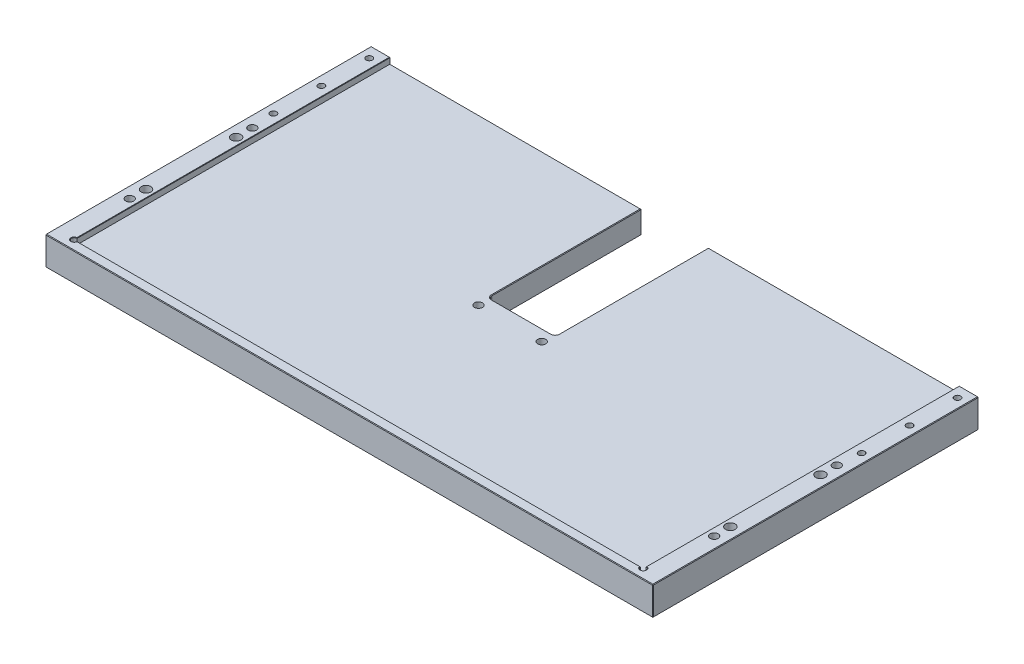
from build123d import *

# Parameters (mm, degrees)
SKETCH_1_W             = 317
SKETCH_1_H             = 170
EXTRUDE_1_DEPTH        = 15
SKETCH_2_W             = 297
SKETCH_2_H             = 330
CUT_EXTRUDE_1_DEPTH    = 3.1
SKETCH_3_W             = 35
SKETCH_3_H             = 103.554222687
CUT_EXTRUDE_2_DEPTH    = 181.477837975
HOLE_WIZARD_M5_1_D     = 4.2
HOLE_WIZARD_M5_1_DEPTH = 16
HOLE_WIZARD_M5_1_TIP   = 1.2618073
FILLET_1_R             = 2
SKETCH_6_R             = 1.5
CUT_EXTRUDE_3_DEPTH    = 5
CHAMFER_1_SIZE         = 0.3
HOLE_WIZARD_M5_2_D     = 4.2
HOLE_WIZARD_M4_1_D     = 3.3
HOLE_WIZARD_M4_1_DEPTH = 13.5
HOLE_WIZARD_M4_1_TIP   = 0.991420021
SKETCH_11_R            = 2.5
CUT_EXTRUDE_4_DEPTH    = 10
SKETCH_12_R            = 1.5
CUT_EXTRUDE_5_DEPTH    = 181.477837975
HOLE_WIZARD_M4_2_D     = 3.3
HOLE_WIZARD_M4_2_DEPTH = 9
HOLE_WIZARD_M4_2_TIP   = 0.991420021
CHAMFER_3_SIZE         = 0.2


with BuildPart() as part:
    # 草图1 → 凸台-拉伸1 (new body)
    with BuildSketch(Plane(origin=(0, 0, 0), x_dir=(1, 0, 0), z_dir=(0, 1, 0))):
        Rectangle(SKETCH_1_W, SKETCH_1_H)
    extrude(amount=EXTRUDE_1_DEPTH)

    # 草图2 → 切除-拉伸1 (cut)
    with BuildSketch(Plane(origin=(0, 15, 0), x_dir=(1, 0, 0), z_dir=(0, 1, 0))):
        with Locations((0, 85)):
            Rectangle(SKETCH_2_W, SKETCH_2_H)
    extrude(amount=-CUT_EXTRUDE_1_DEPTH, mode=Mode.SUBTRACT)

    # 草图3 → 切除-拉伸2 (cut, through all)
    with BuildSketch(Plane.XZ):
        with Locations((0, -56.777111344)):
            Rectangle(SKETCH_3_W, SKETCH_3_H)
    extrude(amount=-CUT_EXTRUDE_2_DEPTH, mode=Mode.SUBTRACT)

    # M5 螺纹孔1
    with Locations(Plane(origin=(0, 0, 0), x_dir=(-1, 0, 0), z_dir=(0, -1, 0))):
        with Locations((-16.5, -1), (16.5, -1)):
            Hole(HOLE_WIZARD_M5_1_D / 2, depth=HOLE_WIZARD_M5_1_DEPTH)
            with Locations((0, 0, -(HOLE_WIZARD_M5_1_DEPTH + HOLE_WIZARD_M5_1_TIP / 2))):  # 118° drill point
                Cone(0, HOLE_WIZARD_M5_1_D / 2, HOLE_WIZARD_M5_1_TIP, mode=Mode.SUBTRACT)

    # 圆角1
    fillet_1_edges = [part.edges().sort_by_distance(p)[0] for p in [
        (17.5, 5.95, -5),
        (-17.5, 5.95, -5),
    ]]
    fillet(fillet_1_edges, radius=FILLET_1_R)

    # 草图6 → 切除-拉伸3 (cut)
    with BuildSketch(Plane(origin=(0, 15, 0), x_dir=(1, 0, 0), z_dir=(0, 1, 0))):
        with Locations(Location((-148.5, -80, 0), (0, 0, 270))):
            Circle(SKETCH_6_R)
        with Locations(Location((148.5, -80, 0), (0, 0, 270))):
            Circle(SKETCH_6_R)
    extrude(amount=-CUT_EXTRUDE_3_DEPTH, mode=Mode.SUBTRACT)

    # 倒角1
    chamfer_1_edges = [part.edges().sort_by_distance(p)[0] for p in [
        (-158.5, 15, 0),
        (0, 15, 85),
        (-153.5, 15, -85),
        (83, 11.9, -85),
        (148.5, 13.45, -85),
        (-148.5, 13.45, -85),
        (-83, 11.9, -85),
        (-17.5, 11.9, -46),
        (-88, 0, -85),
        (17.5, 0, -46),
        (17.5, 5.95, -85),
        (-17.5, 5.95, -85),
        (158.5, 15, 0),
        (0, 0, 85),
        (-158.5, 0, 0),
        (88, 0, -85),
        (158.5, 0, 0),
        (153.5, 15, -85),
        (0, 11.9, -5),
        (0, 0, -5),
        (158.5, 7.5, 85),
        (-158.5, 7.5, 85),
        (17.5, 11.9, -46),
        (-158.5, 7.5, -85),
        (-17.5, 0, -46),
        (158.5, 7.5, -85),
        (16.914213562, 0, -5.585786438),
        (16.914213562, 11.9, -5.585786438),
        (-16.914213562, 0, -5.585786438),
        (-16.914213562, 11.9, -5.585786438),
    ]]
    chamfer(chamfer_1_edges, length=CHAMFER_1_SIZE)

    # M5 螺纹孔2 (through all)
    with Locations(Plane(origin=(0, 15, 0), x_dir=(1, 0, 0), z_dir=(0, 1, 0))):
        with Locations((152.5, 17), (152.5, -47), (-152.5, 17), (-152.5, -47)):
            Hole(HOLE_WIZARD_M5_2_D / 2)

    # M4 螺纹孔1
    with Locations(Plane(origin=(0, 15, 0), x_dir=(1, 0, 0), z_dir=(0, 1, 0))):
        with Locations((153.5, 79), (153.5, 54), (153.5, 29), (-153.5, 29), (-153.5, 54), (-153.5, 79)):
            Hole(HOLE_WIZARD_M4_1_D / 2, depth=HOLE_WIZARD_M4_1_DEPTH)
            with Locations((0, 0, -(HOLE_WIZARD_M4_1_DEPTH + HOLE_WIZARD_M4_1_TIP / 2))):  # 118° drill point
                Cone(0, HOLE_WIZARD_M4_1_D / 2, HOLE_WIZARD_M4_1_TIP, mode=Mode.SUBTRACT)

    # 草图11 → 切除-拉伸4 (cut)
    with BuildSketch(Plane(origin=(0, 15, 0), x_dir=(1, 0, 0), z_dir=(0, 1, 0))):
        with Locations(Location((152.5, 8.5, 0), (0, 0, 270))):
            Circle(SKETCH_11_R)
        with Locations(Location((152.5, -38.5, 0), (0, 0, 270))):
            Circle(SKETCH_11_R)
        with Locations(Location((-152.5, 8.5, 0), (0, 0, 270))):
            Circle(SKETCH_11_R)
        with Locations(Location((-152.5, -38.5, 0), (0, 0, 270))):
            Circle(SKETCH_11_R)
    extrude(amount=-CUT_EXTRUDE_4_DEPTH, mode=Mode.SUBTRACT)

    # 草图12 → 切除-拉伸5 (cut, through all)
    with BuildSketch(Plane(origin=(0, 15, 0), x_dir=(1, 0, 0), z_dir=(0, 1, 0))):
        with Locations(Location((152.5, 8.5, 0), (0, 0, 270))):
            Circle(SKETCH_12_R)
        with Locations(Location((152.5, -38.5, 0), (0, 0, 270))):
            Circle(SKETCH_12_R)
        with Locations(Location((-152.5, 8.5, 0), (0, 0, 270))):
            Circle(SKETCH_12_R)
        with Locations(Location((-152.5, -38.5, 0), (0, 0, 270))):
            Circle(SKETCH_12_R)
    extrude(amount=-CUT_EXTRUDE_5_DEPTH, mode=Mode.SUBTRACT)

    # M4 螺纹孔2
    with Locations(Plane(origin=(0, 0, 0), x_dir=(-1, 0, 0), z_dir=(0, -1, 0))):
        with Locations((148.5, 25), (148.5, -55), (108.5, 25), (108.5, -55), (-148.5, 25), (-108.5, 25), (-148.5, -55), (-108.5, -55)):
            Hole(HOLE_WIZARD_M4_2_D / 2, depth=HOLE_WIZARD_M4_2_DEPTH)
            with Locations((0, 0, -(HOLE_WIZARD_M4_2_DEPTH + HOLE_WIZARD_M4_2_TIP / 2))):  # 118° drill point
                Cone(0, HOLE_WIZARD_M4_2_D / 2, HOLE_WIZARD_M4_2_TIP, mode=Mode.SUBTRACT)

    # 倒角3
    chamfer_3_edges = [part.edges().sort_by_distance(p)[0] for p in [
        (148.5, 15, -3.1),
        (150, 15, 80),
        (-148.5, 15, -3.1),
        (0, 15, 80),
        (-150, 15, 80),
    ]]
    chamfer(chamfer_3_edges, length=CHAMFER_3_SIZE)


solid = part.part
